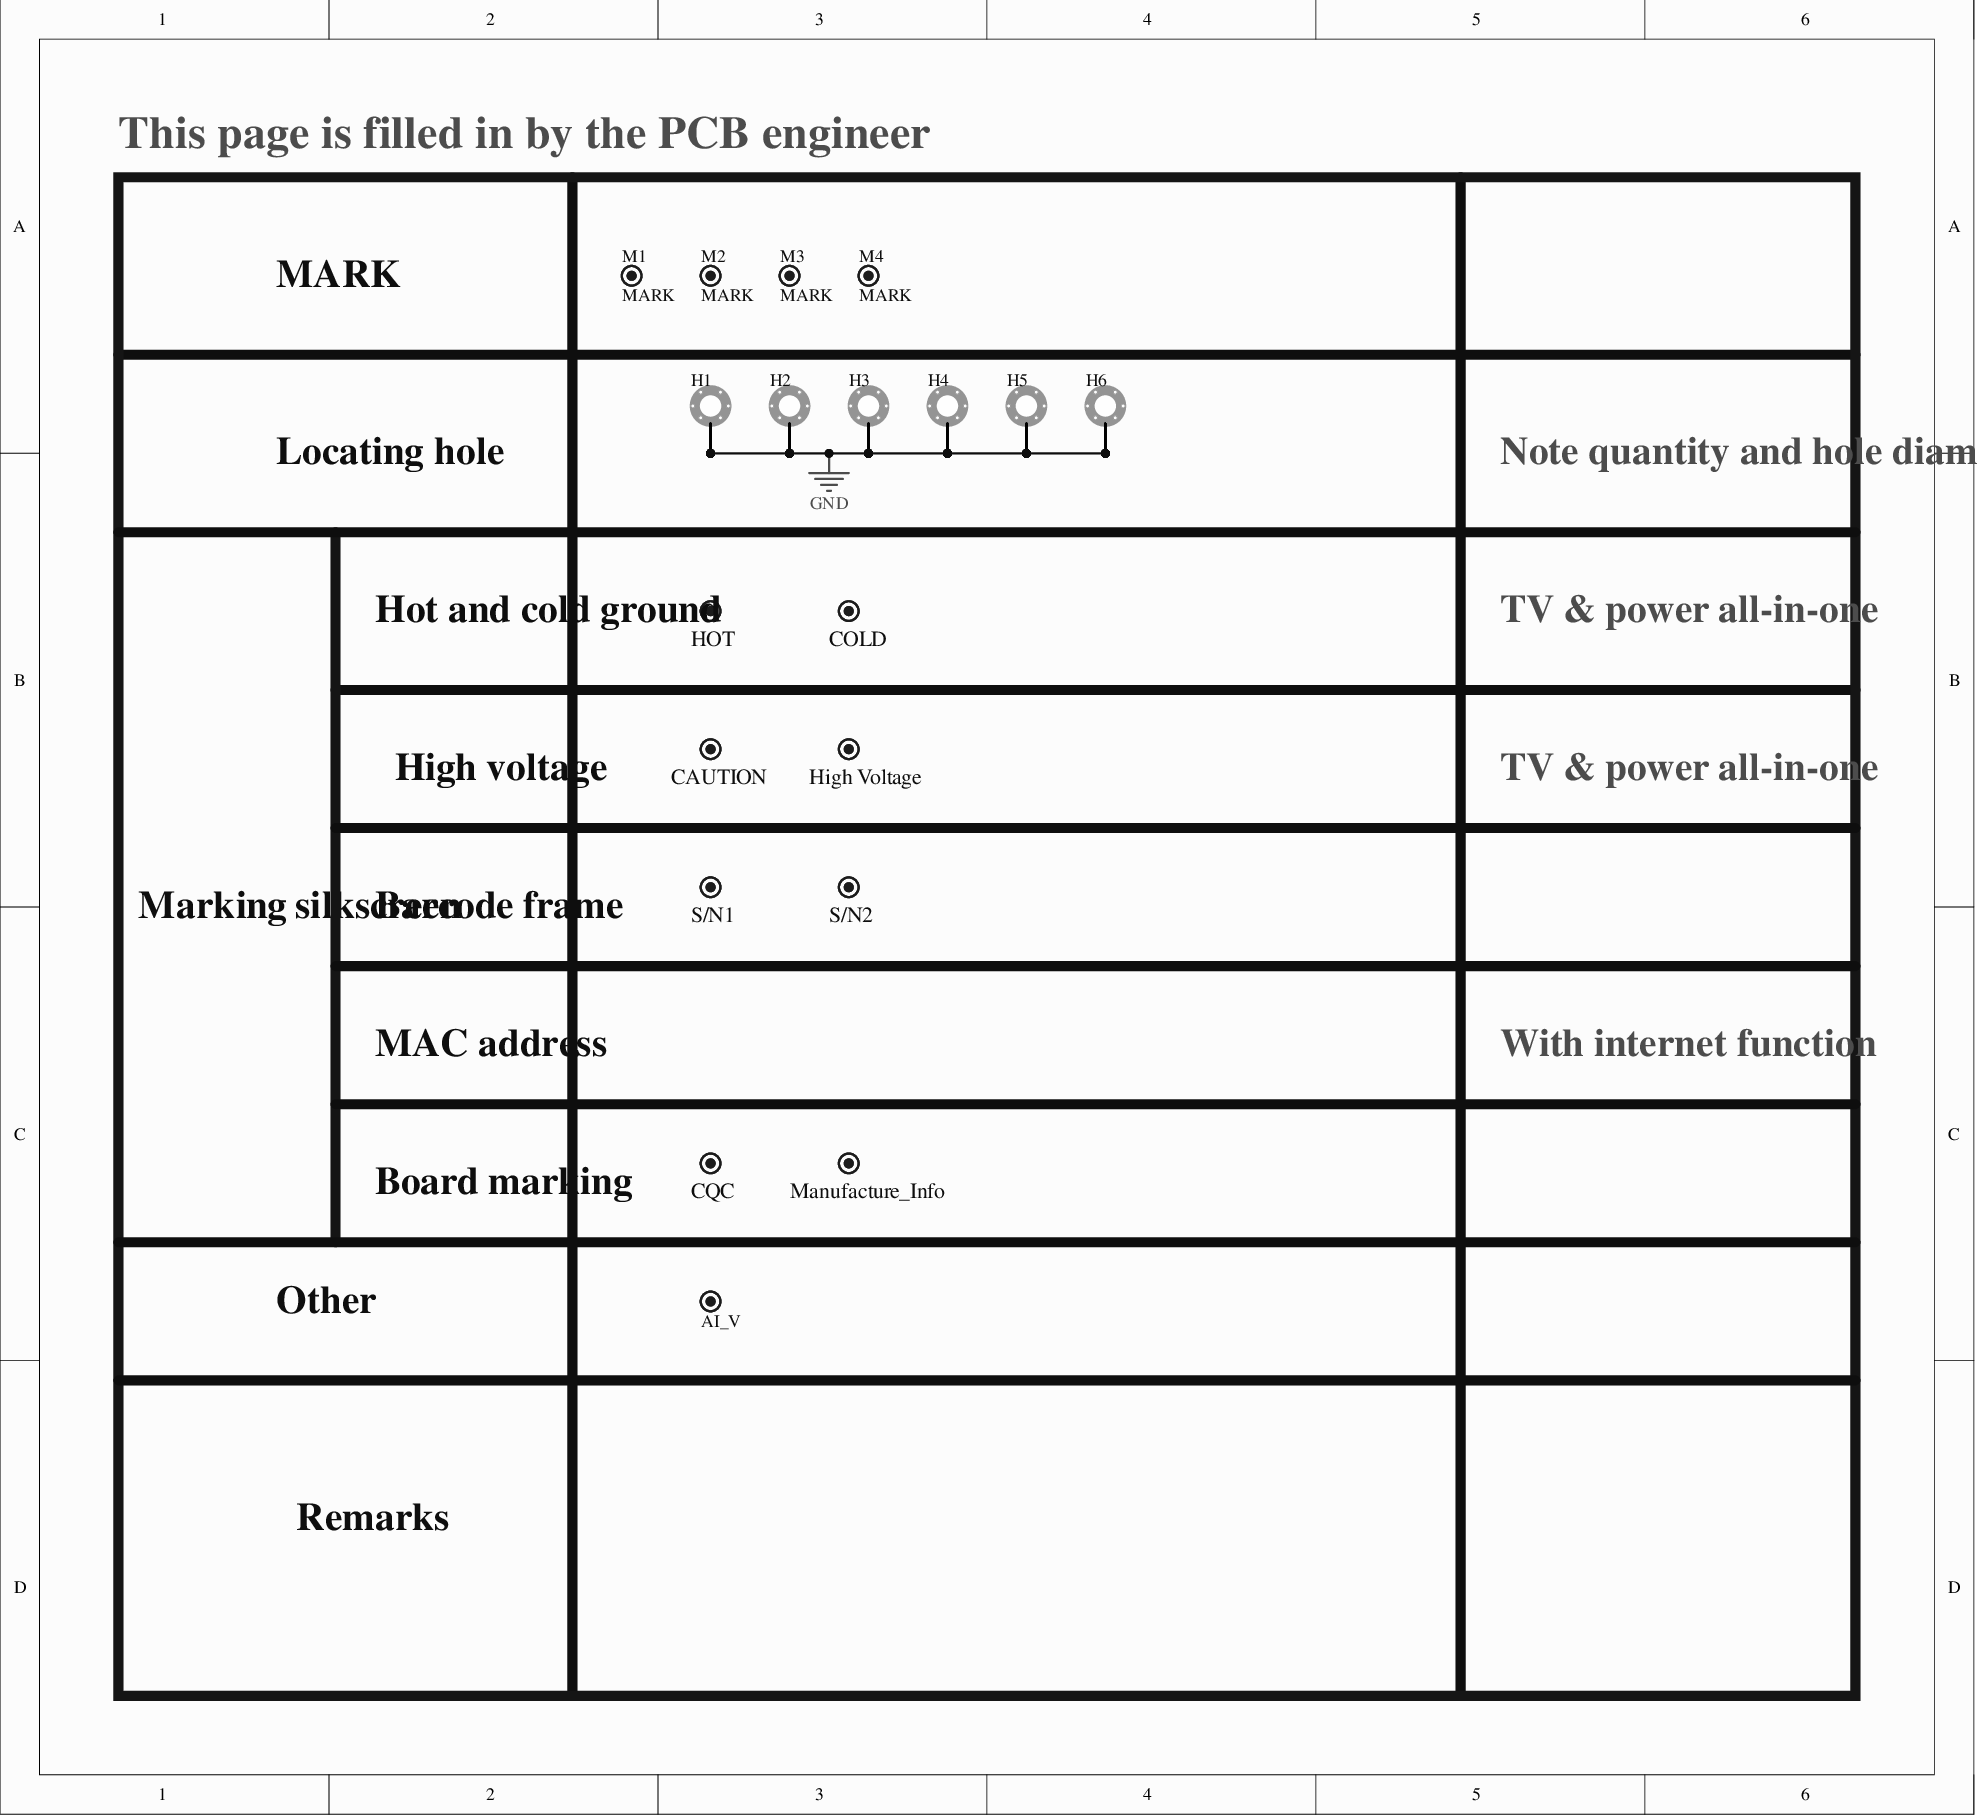
[diagram p0: MISC84438-3.SchDoc]
# Altium project MISC84438-18.PrjPCB (part 1 of 8)
11 sheets, 579 parts. Net scope: global (net labels, ports and power ports of the same name join across sheets).
Board file: MISC84438.PcbDoc
Sheets:
  MISC84438-3.SchDoc
  MISC84438-5.SchDoc
  MISC84438-6.SchDoc
  MISC84438-7.SchDoc
  MISC84438-8.SchDoc
  MISC84438-9.SchDoc
  MISC84438-10.SchDoc
  MISC84438-11.SchDoc
  MISC84438-12.SchDoc
  MISC84438-13.SchDoc
  MISC84438-4.SchDoc

## Sheet MISC84438-3.SchDoc
size 254 x 233 mm

### Parts
AI_V  AI_GRIPPER_V  [AI_GRIPPER_V]  (value not drawn)
CAUTION  CAUTION  [CAUTION]
COLD  COLD  [COLD]
CQC  CQC  [CQC]
H1  Location hole  [ASSE4.0C-3]  (value not drawn)
H2  Location hole  [ASSE4.0C-3]  (value not drawn)
H3  Location hole  [ASSE4.0C-3]  (value not drawn)
H4  Location hole  [ASSE4.0C-3]  (value not drawn)
H5  Location hole  [ASSE4.0C-3]  (value not drawn)
H6  Location hole  [ASSE4.0C-3]  (value not drawn)
High_Voltage  High Voltage  [High Voltage]
HOT  HOT  [HOT]
M1  MARK  [MARK]
M2  MARK  [MARK]
M3  MARK  [MARK]
M4  MARK  [MARK]
Manufacture_Info  Manufacture_Info  [Manufacture_Info]
S/N1  Barcode  [Barcode]  (value not drawn)
S/N2  Barcode  [Barcode]  (value not drawn)

### Nets
GND: H1.1 H1.2 H1.3 H1.4 H1.5 H1.6 H2.1 H2.2 H2.3 H2.4 H2.5 H2.6 H3.1 H3.2 H3.3 H3.4 H3.5 H3.6 H4.1 H4.2 H4.3 H4.4 H4.5 H4.6 H5.1 H5.2 H5.3 H5.4 H5.5 H5.6 H6.1 H6.2 H6.3 H6.4 H6.5 H6.6

### Notes on the sheet
- This page is filled in by the PCB engineer
- MARK
- Locating hole
- Note quantity and hole diameter
- (near HOT) Hot and cold ground
- TV & power all-in-one
- High voltage
- Marking silkscreen
- Barcode frame
- MAC address
- With internet function
- Board marking
- Other
- Remarks

### Library data of the parts
H1-H6 = Location hole-D
M1-M4 = MARK-D

## Sheet MISC84438-5.SchDoc
size 254 x 322 mm
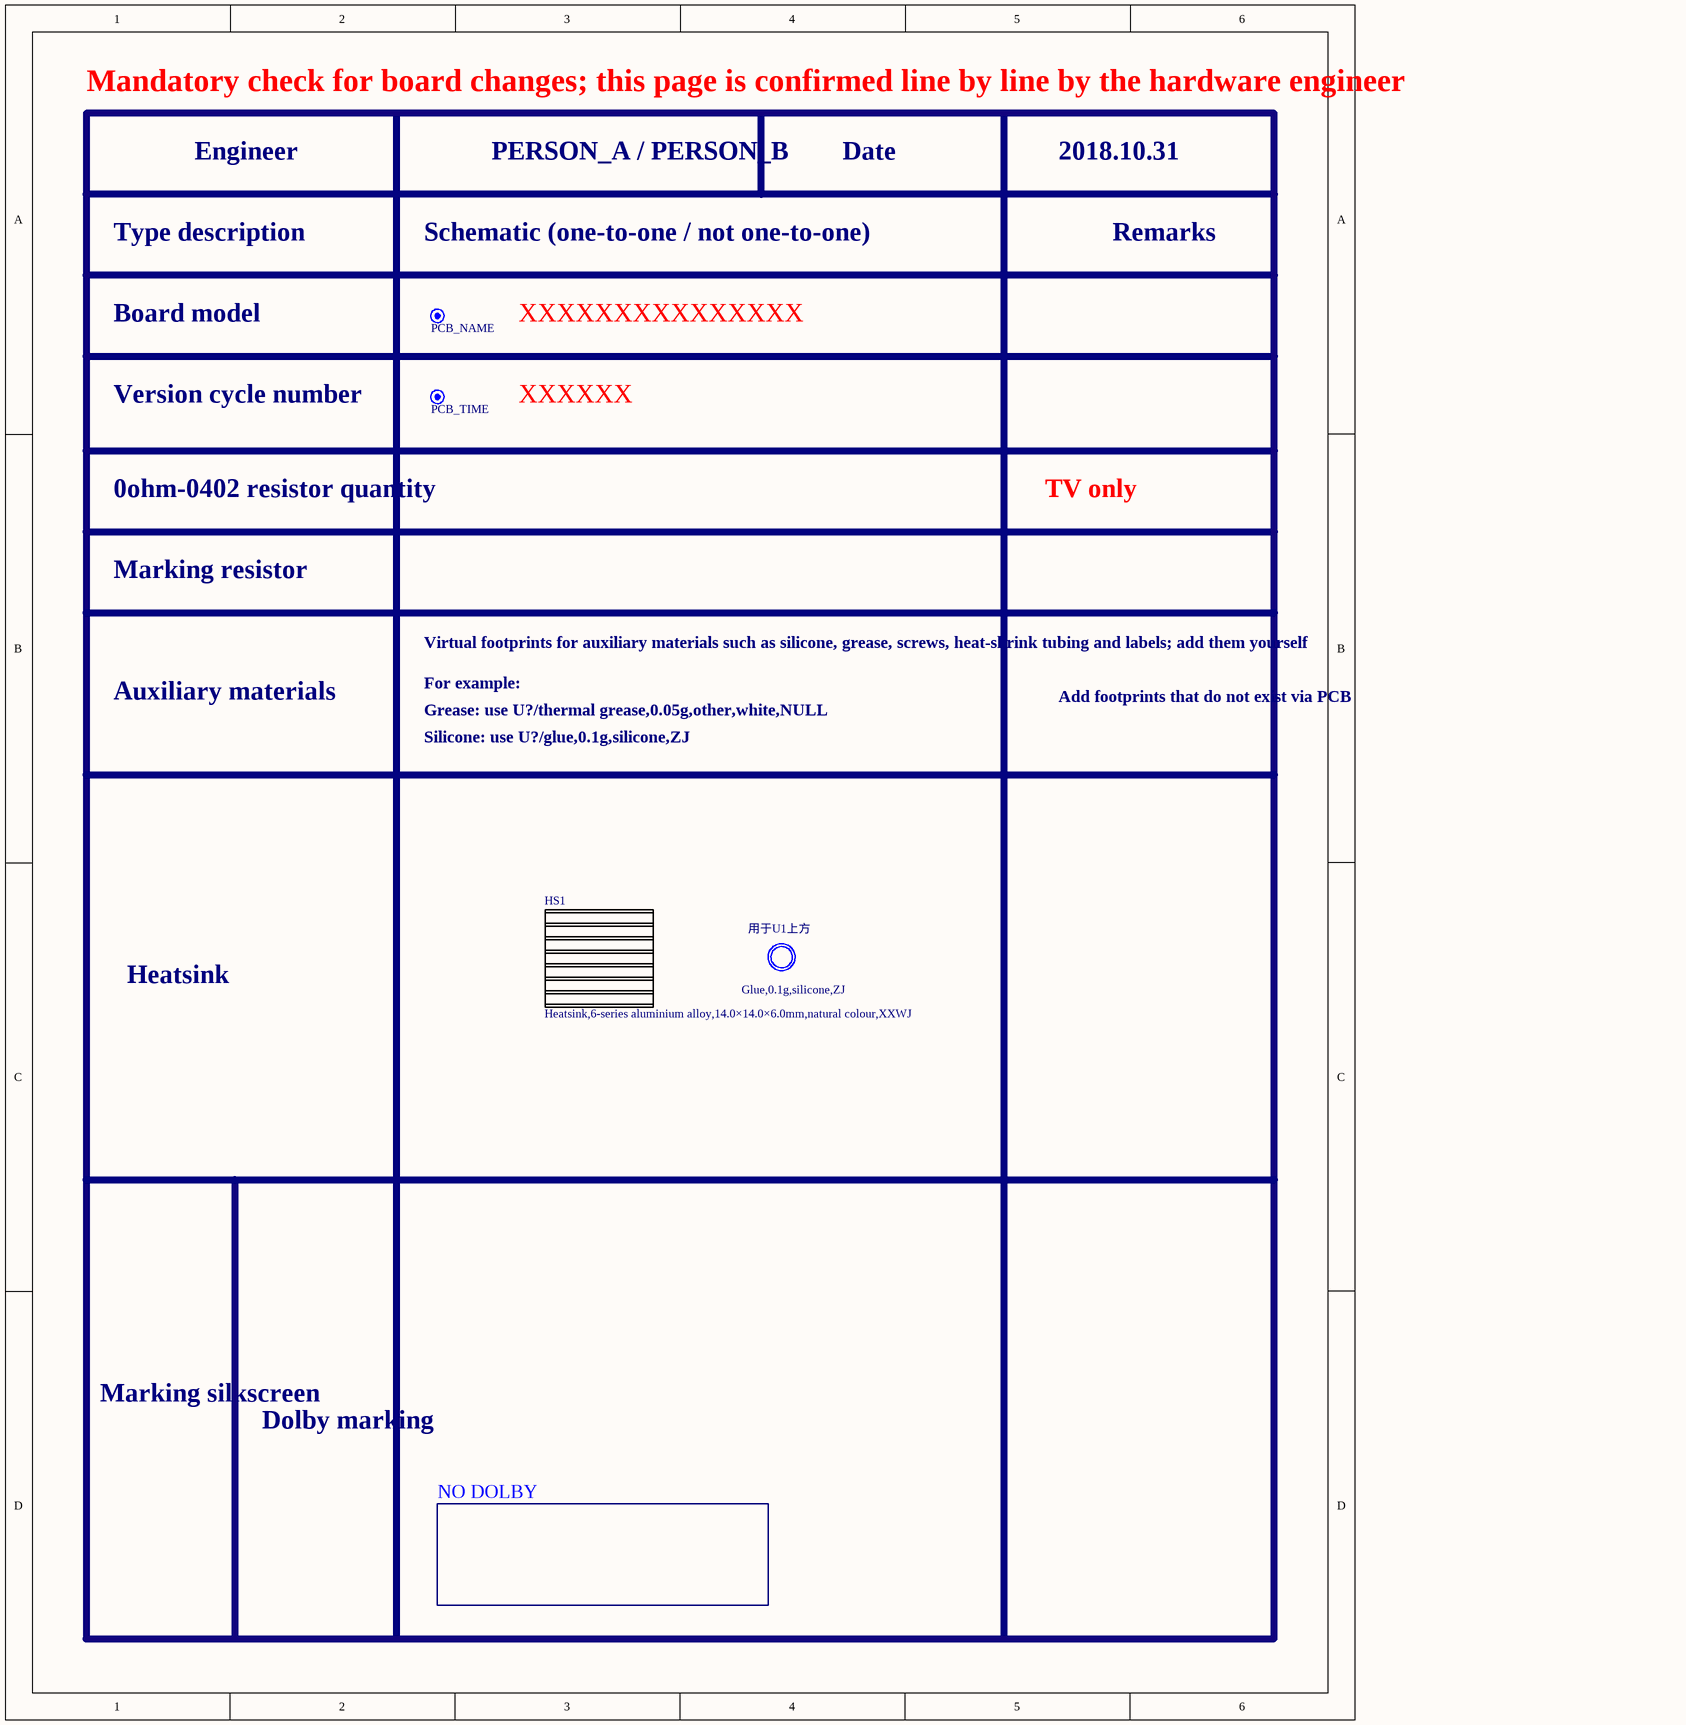
[diagram p1: MISC84438-5.SchDoc]

### Parts
HS1  Heatsink,6-series aluminium alloy,14.0×14.0×6.0mm,natural colour,XXWJ  [HS(14*14*6)]
NO_DOLBY  NO DOLBY  [NO DOLBY-SILK]
XXXXXX  PCB_TIME  [PCB_TIME]
XXXXXXXXXXXXXXX  PCB_NAME  [PCB_NAME]
用于U1上方  Glue,0.1g,silicone,ZJ  [Heat-Shrinkable Tube]

### Notes on the sheet
- Mandatory check for board changes; this page is confirmed line by line by the hardware engineer
- Engineer
- PERSON_A / PERSON_B
- Date
- 2018.10.31
- Type description
- Schematic (one-to-one / not one-to-one)
- Remarks
- Board model
- Version cycle number
- 0ohm-0402 resistor quantity
- TV only
- Marking resistor
- Virtual footprints for auxiliary materials such as silicone, grease, screws, heat-shrink tubing and labels; add them yourself
- Auxiliary materials
- For example:
- Grease: use U?/thermal grease,0.05g,other,white,NULL
- Add footprints that do not exist via PCB
- Silicone: use U?/glue,0.1g,silicone,ZJ
- Heatsink
- Marking silkscreen
- Dolby marking

### Library data of the parts
HS1 = 14×14×06-THD-HS: SMD heatsink
用于U1上方 = Φ12mm×12mm-黑色-125度(UL认证)-D